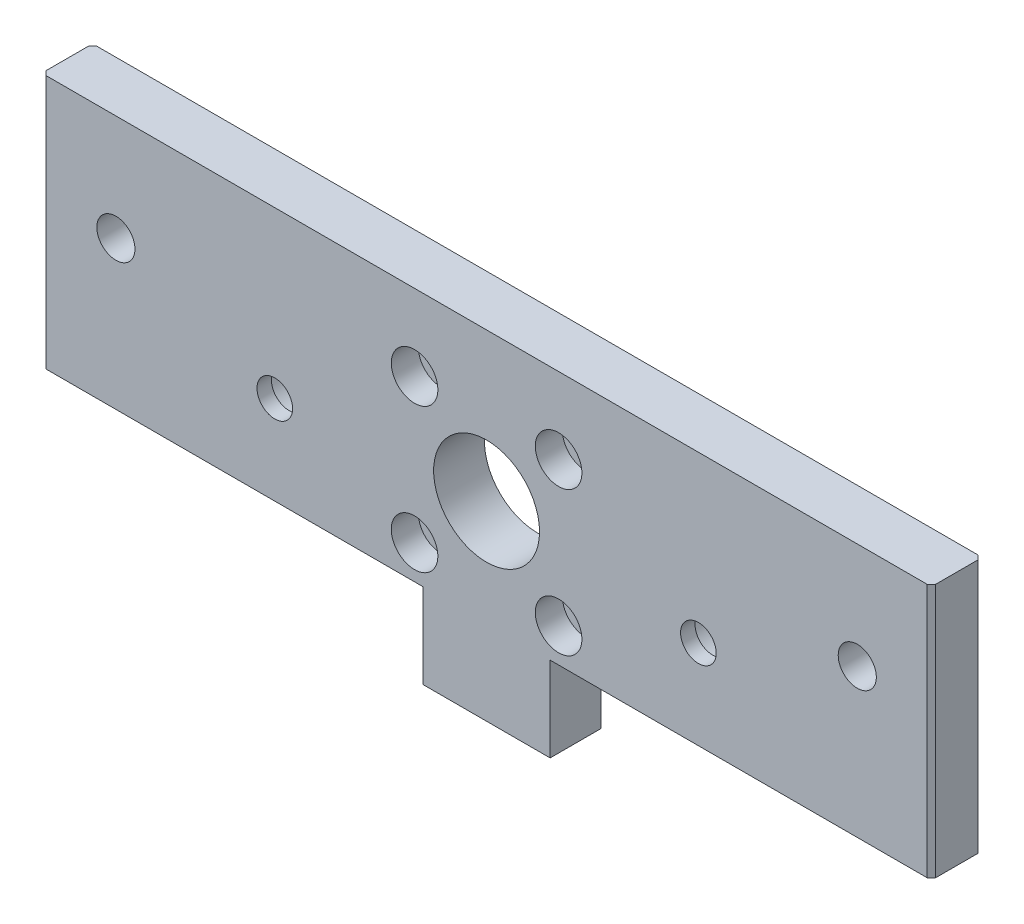
from build123d import *

# Parameters (mm, degrees)
SKETCH_1_W                   = 210
SKETCH_1_H                   = 60
EXTRUDE_1_DEPTH              = 12
SKETCH_2_R                   = 12.5
CUT_EXTRUDE_1_DEPTH          = 12
HOLE_WIZARD_M8_1_D           = 8.4
HOLE_WIZARD_M8_1_CBORE_D     = 15
HOLE_WIZARD_M8_1_CBORE_DEPTH = 8.6
HOLE_WIZARD_M6_2_D           = 6.4
HOLE_WIZARD_M6_2_CBORE_D     = 11
HOLE_WIZARD_M6_2_CBORE_DEPTH = 6.4
CHAMFER_1_SIZE               = 1
HOLE_WIZARD_9_0_9_1_D        = 9
SKETCH_14_W                  = 30
SKETCH_14_H                  = 20
EXTRUDE_2_DEPTH              = 12


with BuildPart() as part:
    # 草图1 → 凸台-拉伸1 (new body)
    with BuildSketch(Plane.XY):
        with Locations((105, 30)):
            Rectangle(SKETCH_1_W, SKETCH_1_H)
    extrude(amount=EXTRUDE_1_DEPTH)

    # 草图2 → 切除-拉伸1 (cut)
    with BuildSketch(Plane.XY.offset(12)):
        with Locations((105, 25)):
            Circle(SKETCH_2_R)
    extrude(amount=-CUT_EXTRUDE_1_DEPTH, mode=Mode.SUBTRACT)

    # M8 六角凹头螺钉的柱形沉头孔1 (through all)
    with Locations(Plane(origin=(0, 0, 0), x_dir=(-1, 0, 0), z_dir=(0, 0, -1))):
        with Locations((-55, 21), (-155, 21)):
            CounterBoreHole(HOLE_WIZARD_M8_1_D / 2, HOLE_WIZARD_M8_1_CBORE_D / 2, HOLE_WIZARD_M8_1_CBORE_DEPTH)

    # M6 六角凹头螺钉的柱形沉头孔2 (through all)
    with Locations(Plane.XY.offset(12)):
        with Locations((122, 42), (88, 42), (122, 8), (88, 8)):
            CounterBoreHole(HOLE_WIZARD_M6_2_D / 2, HOLE_WIZARD_M6_2_CBORE_D / 2, HOLE_WIZARD_M6_2_CBORE_DEPTH)

    # 倒角1
    chamfer_1_edges = [part.edges().sort_by_distance(p)[0] for p in [
        (210, 30, 12),
        (0, 30, 12),
        (210, 30, 0),
        (0, 30, 0),
    ]]
    chamfer(chamfer_1_edges, length=CHAMFER_1_SIZE)

    # Ø9.0 (9) 直径孔1 (through all)
    with Locations(Plane(origin=(0, 0, 0), x_dir=(-1, 0, 0), z_dir=(0, 0, -1))):
        with Locations((-192.5, 35), (-17.5, 35)):
            Hole(HOLE_WIZARD_9_0_9_1_D / 2)

    # 草图14 → 凸台-拉伸2 (add)
    with BuildSketch(Plane(origin=(0, 0, 0), x_dir=(-1, 0, 0), z_dir=(0, 0, -1))):
        with Locations((-105, -10)):
            Rectangle(SKETCH_14_W, SKETCH_14_H)
    extrude(amount=-EXTRUDE_2_DEPTH)


solid = part.part
